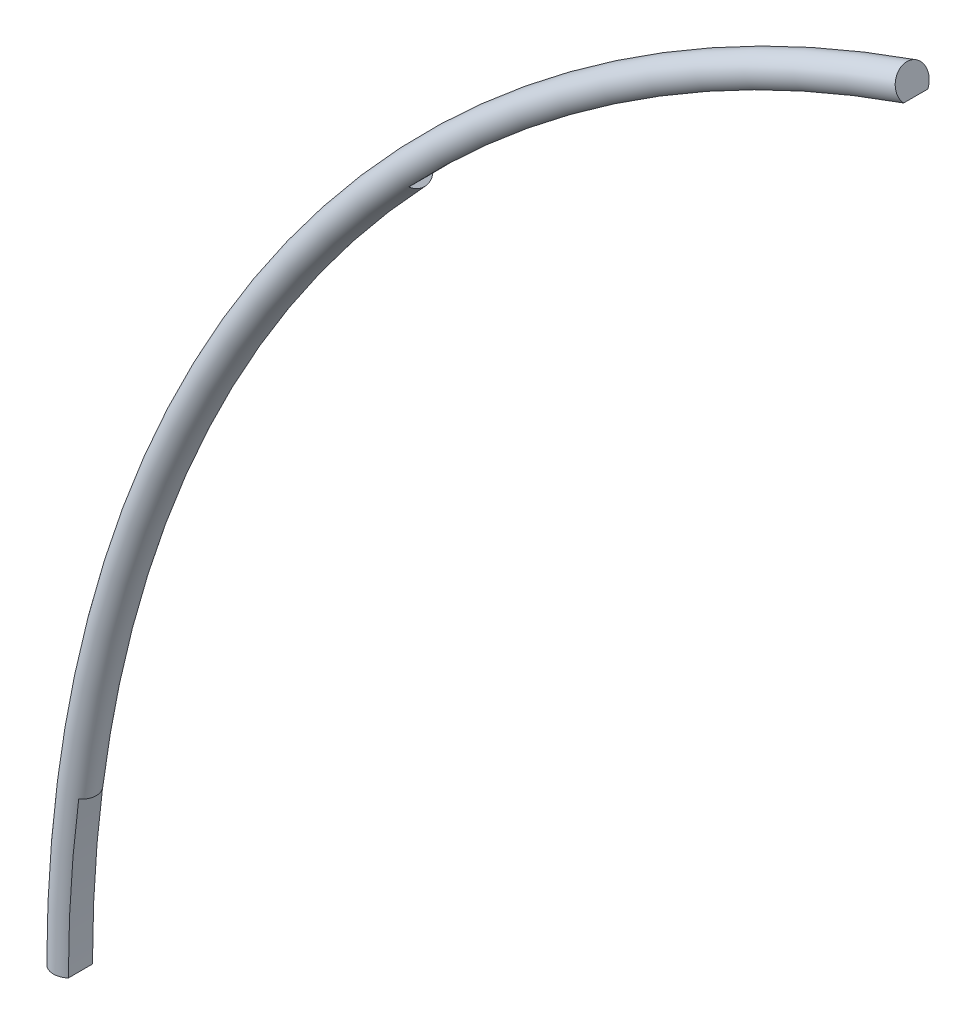
from build123d import *

# Parameters (mm, degrees)
SWEEP1_PROFILE_R   = 3
CUT_EXTRUDE1_DEPTH = 25


with BuildPart() as part:
    # Sweep1: sweep along a path in Sketch1
    with BuildLine(Plane.XY) as sweep1_path:
        ThreePointArc((-76.62592869, 220.039694265), (-189.924776405, 134.972513156), (-233, 0))
    # Sweep1 profile (on start of the path) → Sweep1 (sweep)
    with BuildSketch(Plane(origin=(-76.62592869, 220.039694265, 0), x_dir=(0.3288666467385807, -0.944376370237482, 0), z_dir=(-0.944376370237482, -0.3288666467385807, 0))):
        Circle(SWEEP1_PROFILE_R)
    sweep(path=sweep1_path.line)

    # Sketch6 → Cut-Extrude1 (cut, symmetric)
    with BuildSketch(Plane.XY):
        with BuildLine():
            Line((0, 0), (-229.07603851, 29.751782809))
            ThreePointArc((-229.07603851, 29.751782809), (-230.518507821, 14.906963206), (-231, 0))
            Line((-231, 0), (0, 0))
        make_face()
        with BuildLine():
            Line((0, 0), (-75.968195397, 218.150941525))
            ThreePointArc((-75.968195397, 218.150941525), (-125.473297939, 193.952188707), (-167.838748994, 158.717214996))
            Line((-167.838748994, 158.717214996), (0, 0))
        make_face()
    extrude(amount=CUT_EXTRUDE1_DEPTH, both=True, mode=Mode.SUBTRACT)


solid = part.part
